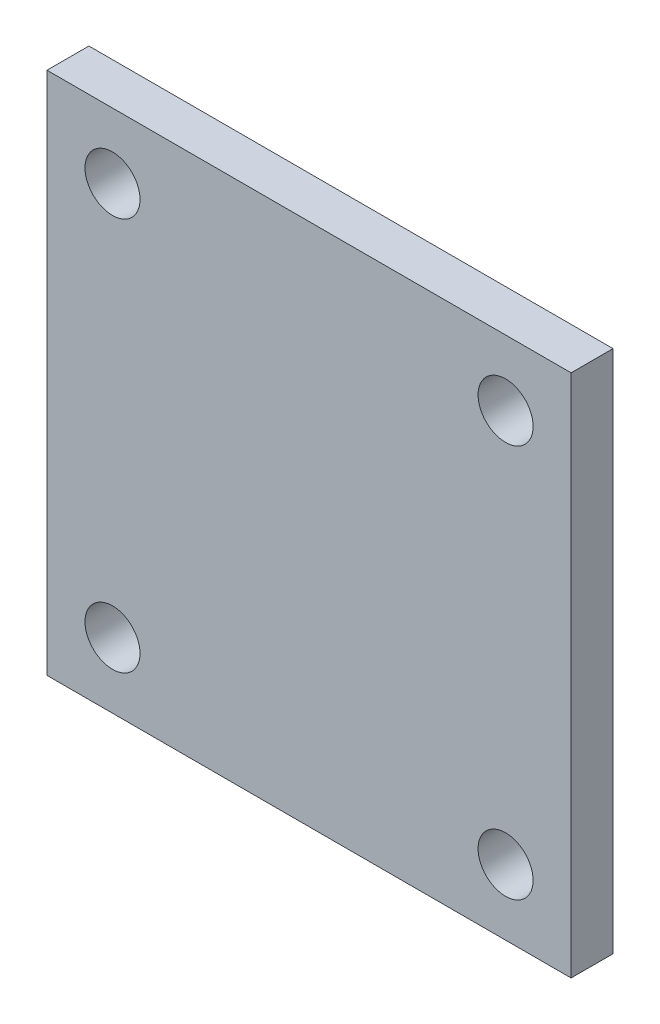
from build123d import *

# Parameters (mm, degrees)
SKETCH1_W      = 200
SKETCH1_H      = 200
EXTRUDE1_DEPTH = 8
SKETCH2_R      = 10.5
EXTRUDE2_DEPTH = 143.323574997


with BuildPart() as part:
    # Sketch1 → Extrude1 (new, symmetric)
    with BuildSketch(Plane.XY):
        Rectangle(SKETCH1_W, SKETCH1_H)
    extrude(amount=EXTRUDE1_DEPTH, both=True)

    # Sketch2 → Extrude2 (cut, through all)
    with BuildSketch(Plane.XY.offset(8)):
        with Locations((-75, 75)):
            Circle(SKETCH2_R)
        with Locations((75, 75)):
            Circle(SKETCH2_R)
        with Locations((-75, -75)):
            Circle(SKETCH2_R)
        with Locations((75, -75)):
            Circle(SKETCH2_R)
    extrude(amount=-EXTRUDE2_DEPTH, mode=Mode.SUBTRACT)


solid = part.part
